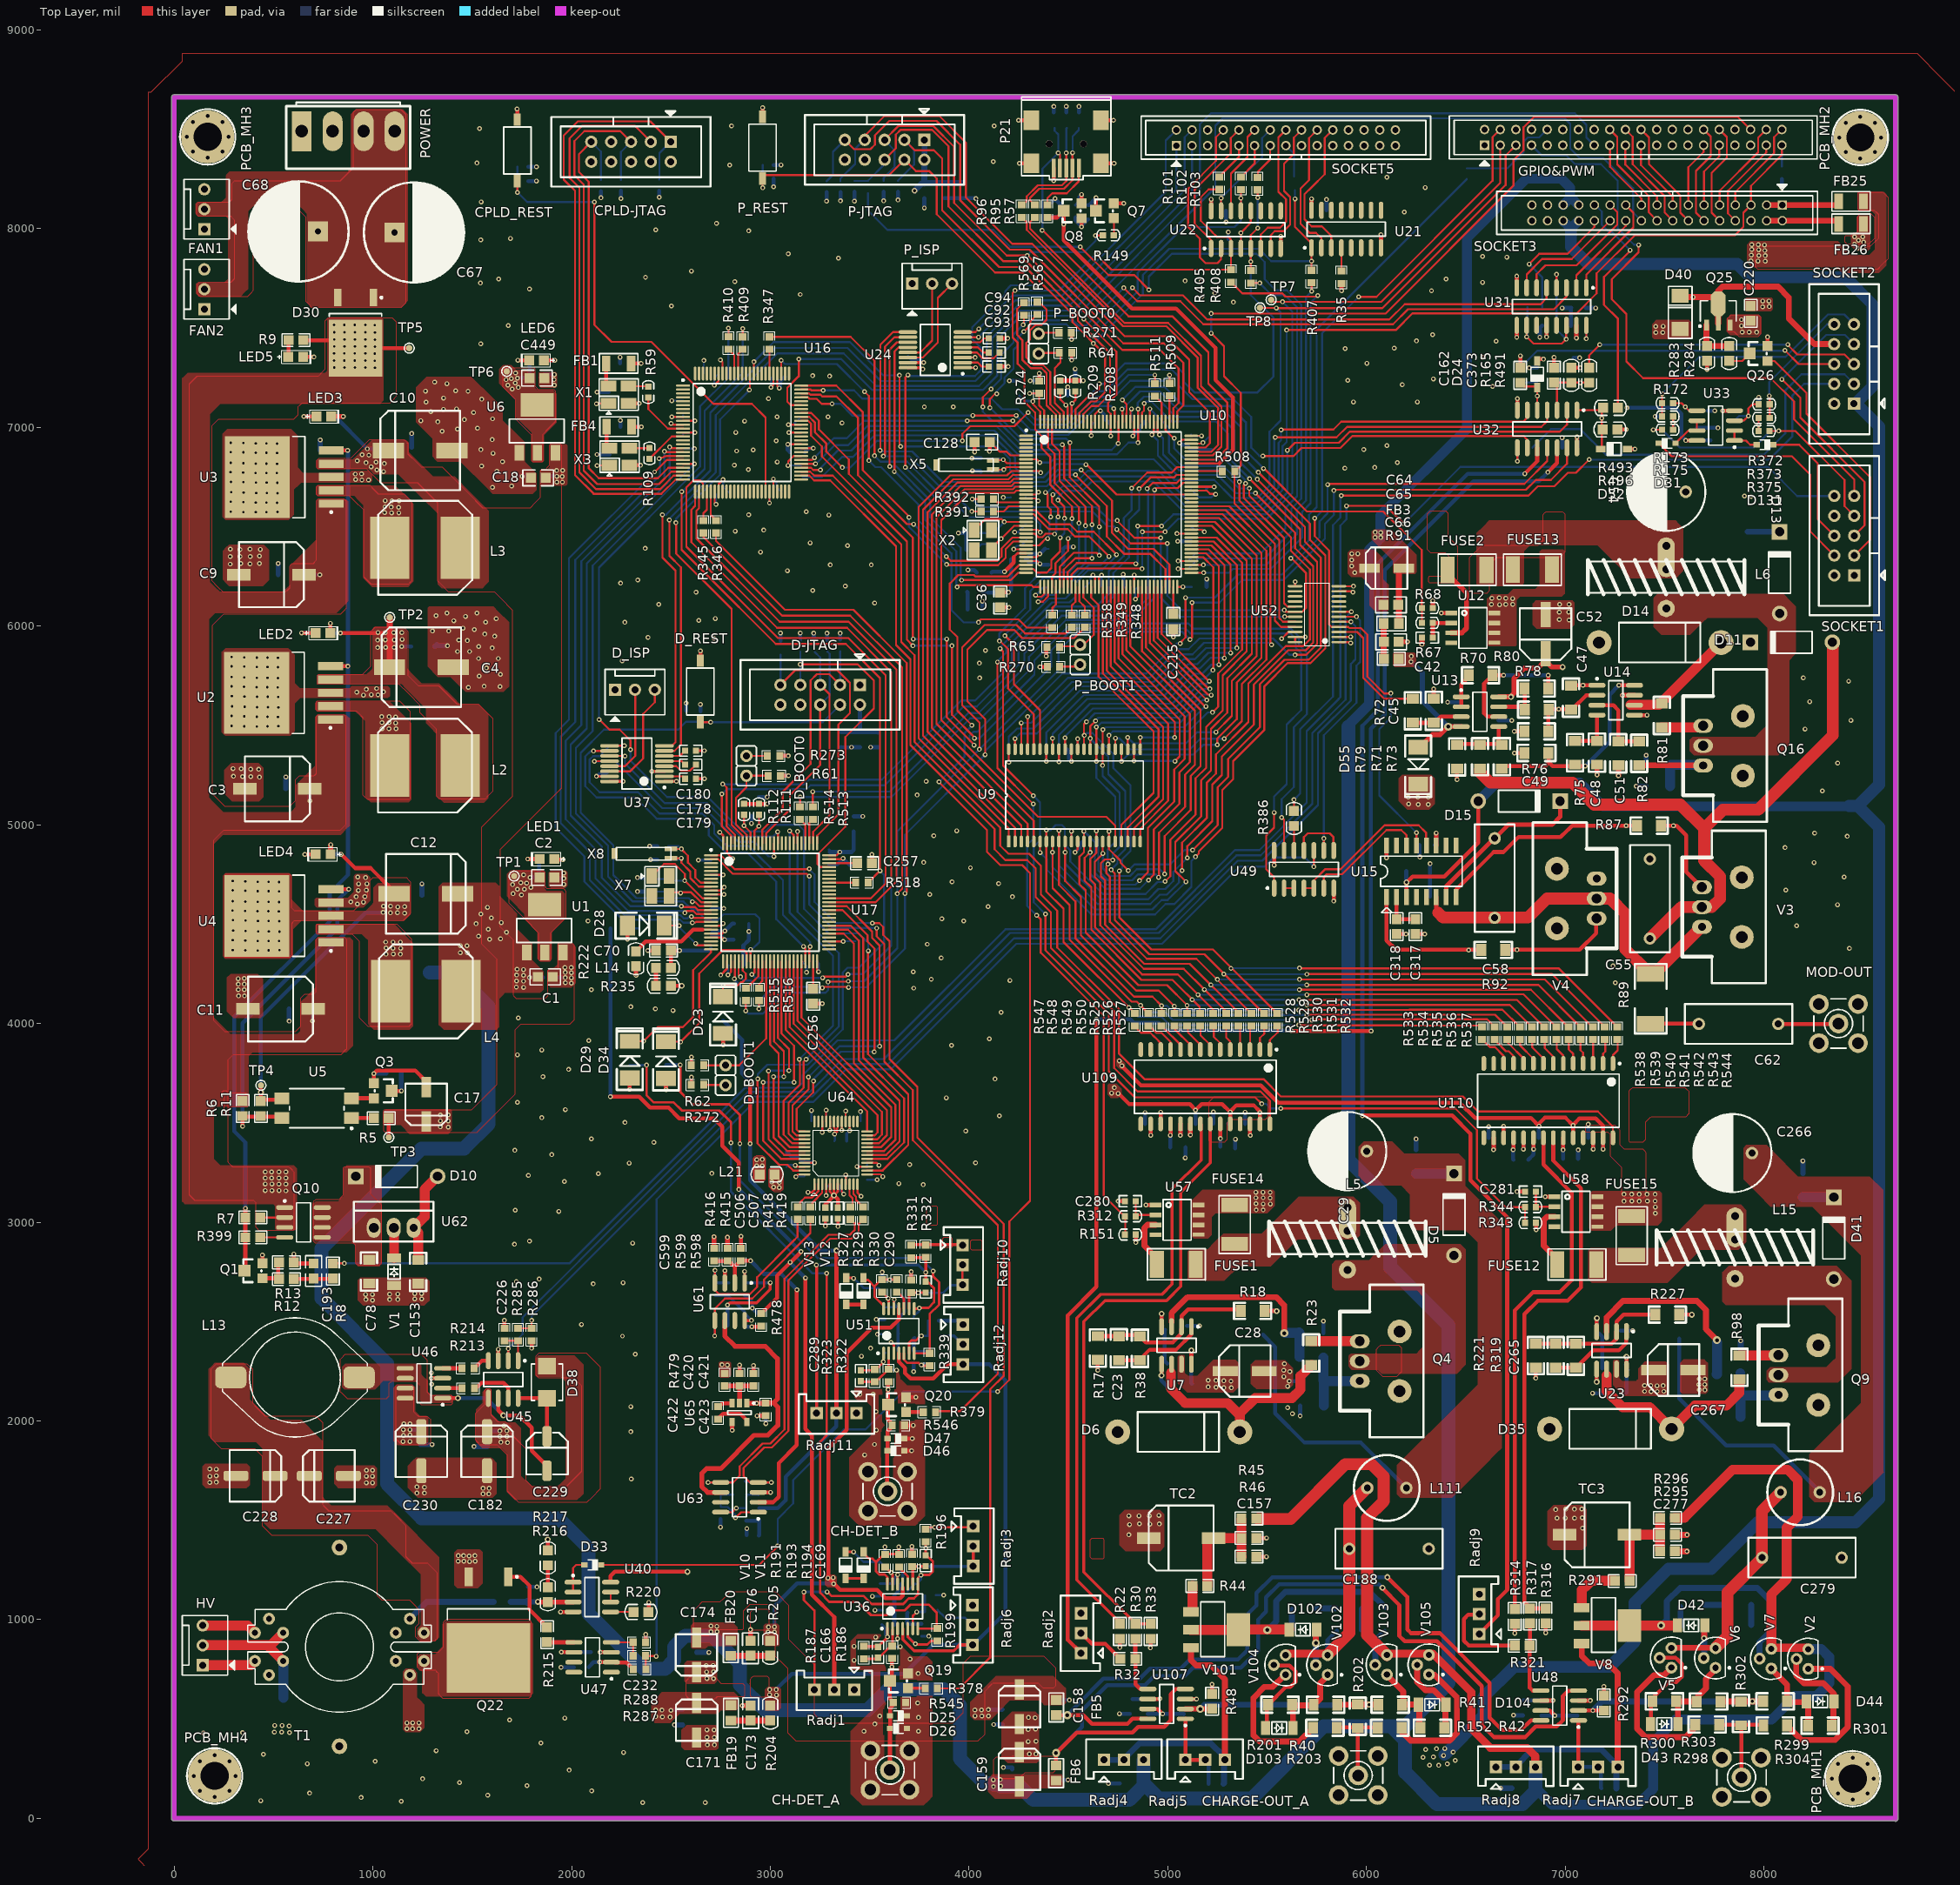
[diagram p0: Top Layer view]
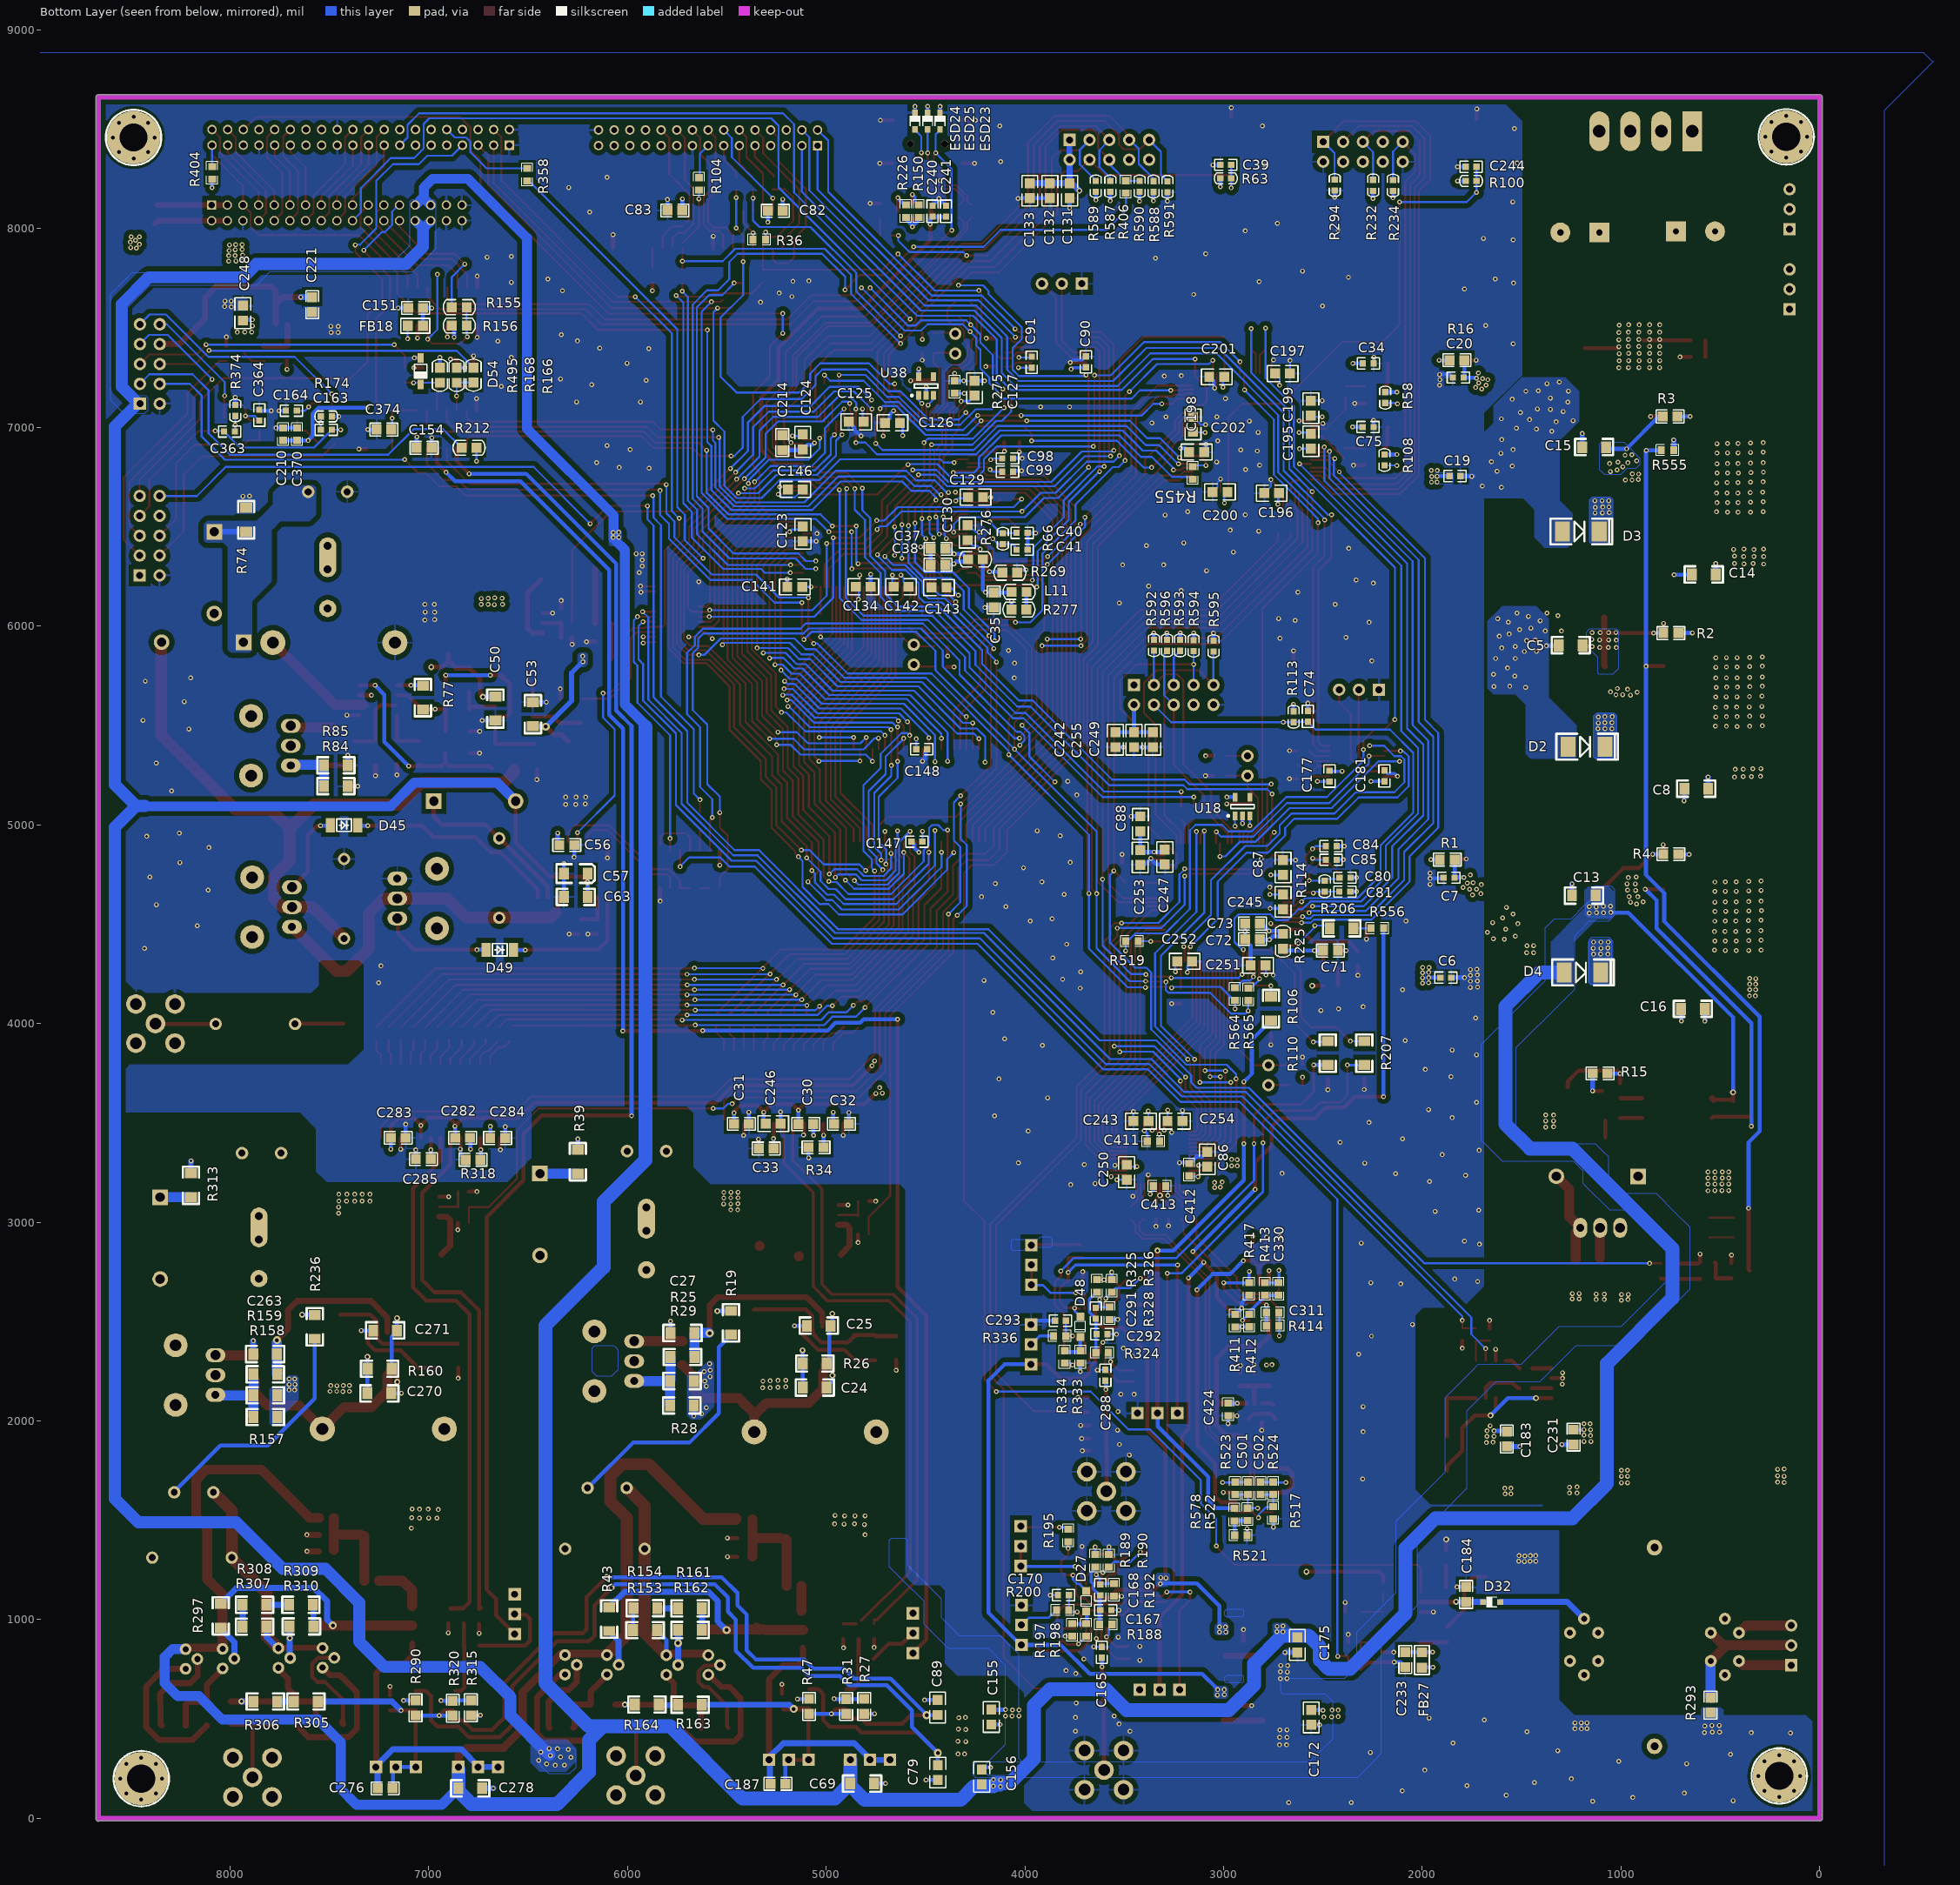
[diagram p1: Bottom Layer view, seen from below]
# Altium PCB MISC82309.PcbDoc (part 1 of 14)
Units mil, origin at the board's own origin, x right, y up, seen from the top; angles counter-clockwise.
Board outline 8687.03 x 8687.86 mil, 4 copper layers (Top Layer, GND, POWER, Bottom Layer); 747 components, 583 nets, 2530 pads, 1834 vias.

## Layer stack, top to bottom (the 12.6 mil dielectric is the usual default, probably not edited)
Top Layer: signal copper 1.4
Dielectric: core 12.6, FR-4, Dk 4.8
GND: plane copper 1.4, net GND
Dielectric: prepreg 12.6, FR-4, Dk 4.8
POWER: plane copper 1.4, net (Multiple Nets)
Dielectric: core 12.6, FR-4, Dk 4.8
Bottom Layer: signal copper 1.4

## Board outline
0,-12.51 cw(c0,0) -12.51,0 -12.51,8661.42 cw(c0,8661.42) 0,8673.93 8661.42,8673.93 cw(c8661.42,8661.42) 8673.26,8665.46 cw(c8662,8660) 8674.51,8660 8674.51,-1.42 cw(c8662,-1.42) 8656.22,-12.51

## Design rules (kind name [scope] priority, off if disabled: settings)
Clearance Clearance_1 [inpolygon] p1: gap=7
Clearance [All] p2: gap=7
DiffPairsRouting [All] p1: maxlimit=10 minlimit=10 mostfreqgap=10 maxuncoupledlength=500
Height [All] p1: minheight=0 maxheight=5000 prefheight=500
HoleSize [All] p1: absolutevalues=TRUE maxlimit=500 minlimit=1 maxpercent=80.000 minpercent=20.000
MinimumSolderMaskSliver [All] p1: minsoldermaskwidth=0
PlaneClearance [All] p1: clearance=20
PlaneConnect [All] p1: planeconnectstyle=Direct reliefexpansion=20 reliefentries=4 reliefconductorwidth=10 reliefairgap=10
PolygonConnect PolygonConnect_1 [All vs isvia] p1: connectstyle=Direct reliefconductorwidth=10 reliefentries=4 polygonreliefangle="90 Angle"
PolygonConnect [All] p2: connectstyle=Relief reliefconductorwidth=10 reliefentries=4 polygonreliefangle="90 Angle"
RoutingVias [All] p1: holewidth=12 width=24 viastyle="Through Hole" minholewidth=12 minwidth=24 maxholewidth=20 maxwidth=40
SilkToSilkClearance [All] p1: silktosilkclearance=0
SilkscreenOverComponentPads [IsPad] p1: minsilkscreentomaskgap=0
SolderMaskExpansion [All] p1: expansion=4
Width [All] p1: maxlimit=100 minlimit=10 preferedwidth=10 minimp=50.000000 maximp=50.000000 favimp=50.000000
20 further rules are at their usual default settings.

## Classes and differential pairs
component class PRINTING_CHARGE_A: C23 C24 C25 C27 C28 C29 C30 C31 C32 C33 C69 C79 C89 C155 C156 C157 C158 C159 C187 C188 C280 CHARGE-OUT_A D5 D6 D102 D103 D104 FB5 FB6 FUSE1 FUSE14 L5 L111 Q4 R17 R18 R19 R22 R23 R25 R26 R27 R28 R29 R30 R31 R32 R33 R34 R38 R39 R40 R41 R42 R43 R44 R45 R46 R47 R48 R151 R152 R153 R154 R161 R162 R163 R164 R201 R202 R203 R312 Radj2 Radj4 Radj5 TC2 U7 U57 U107 U109 V101 V102 V103 V104 V105
component class PRINTING_CHARGE_B: C263 C265 C266 C267 C270 C271 C276 C277 C278 C279 C281 C282 C283 C284 C285 CHARGE-OUT_B D35 D41 D42 D43 D44 FUSE12 FUSE15 L15 L16 Q9 R98 R157 R158 R159 R160 R221 R227 R236 R290 R291 R292 R295 R296 R297 R298 R299 R300 R301 R302 R303 R304 R305 R306 R307 R308 R309 R310 R313 R314 R315 R316 R317 R318 R319 R320 R321 R343 R344 Radj7 Radj8 Radj9 TC3 U23 U48 U58 U110 V2 V5 V6 V7 V8
component class PRINTING_CHARGEDETECT_A: C165 C166 C167 C168 C169 C170 C171 C172 C173 C174 C175 C176 C311 C330 C411 C412 C413 C506 C507 C599 CH-DET_A D25 D26 D27 FB19 FB20 L21 Q19 R186 R187 R188 R189 R190 R191 R192 R193 R194 R195 R196 R197 R198 R199 R200 R204 R205 R378 R411 R412 R413 R414 R415 R416 R417 R418 R419 R478 R545 R556 R598 R599 Radj1 Radj3 Radj6 U36 U61 U64 V10 V11
component class PRINTING_CHARGEDETECT_B: C288 C289 C290 C291 C292 C293 C420 C421 C422 C423 C424 C501 C502 CH-DET_B D46 D47 D48 Q20 R322 R323 R324 R325 R326 R327 R328 R329 R330 R331 R332 R333 R334 R336 R339 R379 R479 R517 R521 R522 R523 R524 R546 R578 Radj10 Radj11 Radj12 U51 U63 U65 V12 V13
component class PRINTING_CONNECT: C82 C83 C90 C91 C92 C93 C94 C177 C178 C179 C180 C181 D_BOOT0 D_BOOT1 D_ISP FB25 FB26 GPIO&PWM P_BOOT0 P_BOOT1 P_ISP R35 R36 R61 R62 R64 R65 R101 R102 R103 R104 R270 R271 R272 R273 R358 R404 SOCKET1 SOCKET2 SOCKET3 SOCKET5 TP7 TP8 U21 U22 U24 U37
component class PRINTING_CPLD: C34 C75 C195 C196 C197 C198 C199 C200 C201 C202 C244 CPLD-JTAG CPLD_REST FB1 FB4 R58 R59 R100 R108 R109 R232 R234 R294 R345 R346 R347 R409 R410 R455 R558 U16 X1 X3
component class PRINTING_HV: C182 C183 C184 C226 C227 C228 C229 C230 C231 C232 C233 D32 D33 D38 FB27 HV L13 Q22 R213 R214 R215 R216 R217 R220 R285 R286 R287 R288 R293 T1 U40 U45 U46 U47
component class PRINTING_MCU_DECTECT: C70 C71 C72 C73 C74 C80 C81 C84 C85 C86 C87 C88 C242 C243 C245 C246 C247 C248 C249 C250 C251 C252 C253 C254 C255 C256 C257 D23 D28 D29 D34 D-JTAG D_REST L14 R106 R110 R111 R112 R113 R114 R206 R207 R222 R225 R235 R513 R514 R515 R516 R518 R519 R564 R565 R592 R593 R594 R595 R596 U17 U18 X7 X8
component class PRINTING_MCU_PROCESSOR: C35 C36 C37 C38 C39 C40 C41 C98 C99 C123 C124 C125 C126 C127 C128 C129 C130 C131 C132 C133 C134 C141 C142 C143 C146 C214 C215 C240 C241 ESD23 ESD24 ESD25 L11 P21 P-JTAG P_REST Q7 Q8 R57 R63 R66 R95 R96 R149 R150 R208 R209 R226 R269 R274 R275 R276 R277 R348 R349 R391 R392 R405 R406 R407 R408 R508 R509 R511 R567 R569 R587 R588 R589 R590 R591 U10 U38 X2 X5
component class PRINTING_MODULATION: C42 C45 C47 C48 C49 C50 C51 C52 C53 C54 C55 C56 C57 C58 C62 C63 C64 C65 C66 C317 C318 D11 D13 D14 D15 D45 D49 D55 FB3 FUSE2 FUSE13 L6 MOD-OUT Q16 R67 R68 R70 R71 R72 R73 R74 R75 R76 R77 R78 R79 R80 R81 R82 R84 R85 R87 R89 R91 R92 U12 U13 U14 U15 U49 U52 V3 V4
component class PRINTING_SYNCHRONIZER: C151 C154 C162 C163 C164 C210 C220 C221 C363 C364 C370 C373 C374 D24 D31 D40 D52 D54 D131 FB18 Q25 Q26 R155 R156 R165 R166 R168 R172 R173 R174 R175 R212 R283 R284 R372 R373 R374 R375 R386 R491 R493 R495 R496 U31 U32 U33
component class SYSTEM_POWER: C1 C2 C3 C4 C5 C6 C7 C8 C9 C10 C11 C12 C13 C14 C15 C16 C17 C18 C19 C20 C67 C68 C78 C153 C193 C449 D2 D3 D4 D10 D30 FAN1 FAN2 L2 L3 L4 LED1 LED2 LED3 LED4 LED5 LED6 PCB_MH1 PCB_MH2 PCB_MH3 PCB_MH4 POWER Q1 Q3 Q10 R1 R2 R3 R4 R5 R6 R7 R8 R9 R11 R12 R13 R15 R16 R399 R555 TP1 TP2 TP3 TP4 TP5 TP6 U1 U2 U3 U4 U5 U6 U62 V1
net class D_A[0..11]: D_A0 D_A1 D_A2 D_A3 D_A4 D_A5 D_A6 D_A7 D_A8 D_A9 D_A10 D_A11
net class D_B[0..11]: D_B0 D_B1 D_B2 D_B3 D_B4 D_B5 D_B6 D_B7 D_B8 D_B9 D_B10 D_B11
net class DET_D[0..15]: DET_D0 DET_D1 DET_D2 DET_D3 DET_D4 DET_D5 DET_D6 DET_D7 DET_D8 DET_D9 DET_D10 DET_D11 DET_D12 DET_D13 DET_D14 DET_D15
net class FSMC_A[0..25]: FSMC_A0 FSMC_A1 FSMC_A2 FSMC_A3 FSMC_A4 FSMC_A5 FSMC_A6 FSMC_A7 FSMC_A8 FSMC_A9 FSMC_A10 FSMC_A11 FSMC_A12 FSMC_A13 FSMC_A14 FSMC_A15 FSMC_A16 FSMC_A17 FSMC_A18 FSMC_A19 FSMC_A20 FSMC_A21 FSMC_A22 FSMC_A23 FSMC_A24 FSMC_A25
net class FSMC_D[0..15]: FSMC_D0 FSMC_D1 FSMC_D2 FSMC_D3 FSMC_D4 FSMC_D5 FSMC_D6 FSMC_D7 FSMC_D8 FSMC_D9 FSMC_D10 FSMC_D11 FSMC_D12 FSMC_D13 FSMC_D14 FSMC_D15
component class PRINTING_RAM: C147 C148 R525 R526 R527 R528 R529 R530 R531 R532 R533 R534 R535 R536 R537 R538 R539 R540 R541 R542 R543 R544 R547 R548 R549 R550 U9
differential pair NewDifferentialPair1: +OUT- -OUT+

## Components (designator, comment, footprint, x,y, rotation, side; value= is the part's Value field where it differs from the comment)
C1 "22uF" C0805 1868,4235 r0 top
C2 "22uF" C0805 1876,4735 r180 top
C3 "220uF/35V" E8X10,2 683,5181 r180 top
C4 "470uF/25V" E10X10.2 1084,5793 r0 top
C5 "0.1uF" C1206 1253,5903 r0 bottom
C6 "0.1uF" C0603 1882,4231 r0 bottom
C7 "0.1uF" C0603 1866,4734 r180 bottom
C8 "0.1uF" C1206 622,5181 r0 bottom
C9 "220uF/35V" E8X10,2 653,6259 r180 top
C10 "470uF/25V" E10X10.2 1078,6884 r0 top
C11 "220uF/35V" E8X10,2 699,4073 r180 top
C12 "470uF/25V" E10X10.2 1427,4653 r180 top
C13 "0.1uF" C1206 1187,4645 r180 bottom
C14 "0.1uF" C1206 584,6259 r0 bottom
C15 "0.1uF" C1206 1136,6900 r0 bottom
C16 "0.1uF" C1206 639,4073 r0 bottom
C17 "47uF/16V" E5X5.4 1269,3507 r90 top
C18 "22uF" C0805 1832,6746 r0 top
C19 "0.1uF" C0603 1836,6755 r0 bottom
C20 "0.1uF" C0603 1819,7251 r180 bottom
C23 "47pF" C1206 4755,2366 r270 top
C24 "10nF" C1206 5057,2169 r180 bottom
C25 "2.2nF" C1206 5037,2479 r0 bottom
C27 "470pF" C1206 5723,2442 r0 bottom
C28 "22uF/35V" E6.3X5.4 5289,2251 r0 top
C29 "2.2uF/450V" CAP-EL-10X13_5-5 5903,3358 r0 top
C30 "0.1uF" CAP_0805 5102,3494 r180 bottom
C31 "0.1uF" CAP_0805 5426,3495 r180 bottom
C32 "0.1uF" CAP_0805 4923,3495 r180 bottom
C33 "0.1uF" CAP_0805 5301,3371 r180 bottom
C34 "0.1uF" C0603 2272,7322 r0 bottom
C35 "1uF" CAP_0805 4157,6131 r90 bottom
C36 "0.1uF" CAP_0805 4157,6131 r90 top
C37 "1uF" CAP_0805 4437,6389 r180 bottom
C38 "0.1uF" CAP_0805 4437,6309 r180 bottom
C39 "0.1uF" C0603 2989,8321 r180 bottom
C40 "20pF" C0603 4014,6469 r0 bottom
C41 "20pF" C0603 4014,6384 r0 bottom
C42 "470pF" C0603 6306,5942 r0 top
C45 "0.22uF" c1206 6338,5574 r90 top
C47 "47pF" C1206 7030,5640 r270 top
C48 "2.2nF" C1206 7160,5363 r270 top
C49 "10nF" C1206 6855,5361 r180 top
C50 "0.47uF" c1206 6664,5585 r270 bottom
C51 "470pF" C1206 7268,5360 r270 top
C52 "22uF/35V" E6.3X5.4 6901,5861 r90 top
C53 "0.47uF" c1206 6476,5557 r90 bottom
C54 "2.2uF/450V" CAP-EL-10X13_5-5 7508,6676 r0 top
C55 "0.33uF/400V" CBB-400V-10mm 7426,4628 r270 top
C56 "0.1uF" CAP_0805 6305,4898 r180 bottom
C57 "22uF/35V" CAP_AVX-A 6260,4755 r0 bottom
C58 "0.1uF/400V" CBB-400V-10mm 6645,4732 r90 top
C62 "22nF/630V" CBB-400V-10mm 7872,3998 r0 top
C63 "0.1uF" C1206 6260,4638 r180 bottom
C64 "10uF/25V" E5X5.4 6015,6291 r0 top
C65 "0.1uF" C0805 6123,6107 r0 top
C66 "0.1uF" C0805 6124,5921 r180 top
C67 "1000uF/35V" CAP-EL-12x20 1207,7981 r0 top
C68 "1000uF/35V" CAP-EL-12x20 626,7986 r180 top
C69 "0.47uF" C1206 4819,176 r180 bottom
C70 "1uF" CAP_0805 2462,4367 r0 top
C71 "0.1uF" CAP_0805 2462,4367 r0 bottom
C72 "1uF" CAP_0805 2855,4425 r180 bottom
C73 "0.1uF" CAP_0805 2855,4503 r180 bottom
C74 "0.1uF" C0603 2576,5546 r270 bottom
C75 "0.1uF" C0603 2273,7002 r0 bottom
C78 "0.33uF" c1206 982,2752 r270 top
C79 "0.1uF" C0805 4438,231 r90 bottom
C80 "20pF" C0603 2389,4734 r0 bottom
C81 "20pF" C0603 2390,4664 r0 bottom
C82 "0.1uF" CAP_0805 5256,8090 r180 bottom
C83 "0.1uF" CAP_0805 5761,8092 r180 bottom
C84 "10pF" C0603 2459,4893 r0 bottom
C85 "10pF" C0603 2459,4824 r0 bottom
C86 "100nF" C0805 3082,3317 r270 bottom
C87 "100nF" C0805 2701,4785 r270 bottom
C88 "100nF" C0805 3419,5005 r270 bottom
C89 "0.1uF" C0805 4439,558 r270 bottom
C90 "0.1uF" C0603 3693,7330 r270 bottom
C91 "0.1uF" C0603 3966,7328 r270 bottom
C92 "0.1uF" C0603 4126,7377 r0 top
C93 "0.1uF" C0603 4126,7306 r180 top
C94 "0.1uF" C0603 4127,7448 r180 top
C98 "10pF" C0603 4087,6844 r0 bottom
C99 "10pF" C0603 4087,6777 r0 bottom
C123 "10uF" C0805 5117,6464 r90 bottom
C124 "100nF" C0805 5118,6927 r90 bottom
C125 "10uF" C0805 4849,7028 r180 bottom
C126 "100nF" C0805 4666,7023 r180 bottom
C127 "10uF" C0805 4253,7197 r270 bottom
C128 "100nF" C0805 4066,6926 r0 top
C129 "10uF" C0805 4248,6649 r0 bottom
C130 "100nF" C0805 4289,6470 r270 bottom
C131 "10uF" C0805 3775,8191 r90 bottom
C132 "100nF" C0805 3874,8191 r90 bottom
C133 "10uF" C0805 3975,8191 r90 bottom
C134 "100nF" C0805 4813,6198 r0 bottom
C141 "10uF" C0805 5158,6197 r180 bottom
C142 "100nF" C0805 4623,6198 r0 bottom
C143 "10uF" C0805 4432,6194 r0 bottom
C146 "100nF" C0805 5155,6688 r0 bottom
C147 "100nF" C0603 4543,4915 r180 bottom
C148 "100nF" C0603 4519,5381 r0 bottom
C151 "0.1uF" CAP_0805 7066,7601 r180 bottom
C153 "0.1uF" c1206 1229,2750 r270 top
C154 "0.1uF" CAP_0805 7023,6897 r0 bottom
C155 "100nF" C0805 4169,510 r270 bottom
C156 "100nF" C0805 4217,209 r90 bottom
C157 "0.1uF" CAP_0805 5408,1317 r0 top
C158 "10uF/25V" E5X5.4 4253,648 r270 top
C159 "10uF/25V" E5X5.4 4253,333 r270 top
C162 "0.1uF" CAP_0805 6774,7262 r270 top
C163 "0.47uF" C0603 7515,6988 r180 bottom
C164 "330pF" C0603 7691,7084 r180 bottom
C165 "470pF" C0603 3613,836 r270 bottom
C166 "1.5nF" C0603 3542,836 r270 top
C167 "0.01uF" C0603 3593,1048 r180 bottom
C168 "0.01uF" C0603 3621,1150 r270 bottom
C169 "1.5nF" C0603 3782,1297 r270 top
C170 "0.22uF" C0603 3806,1124 r0 bottom
C171 "10uF/25V" E5X5.4 2629,580 r270 top
C172 "0.1uF" C0805 2559,508 r90 bottom
C173 "0.1uF" C0805 2901,530 r270 top
C174 "10uF/25V" E5X5.4 2629,737 r90 top
C175 "0.1uF" C0805 2629,873 r90 bottom
C176 "0.1uF" C0805 2900,856 r270 top
C177 "0.1uF" C0603 2467,5245 r270 bottom
C178 "0.1uF" C0603 2599,5303 r0 top
C179 "0.1uF" C0603 2599,5232 r180 top
C180 "0.1uF" C0603 2599,5373 r180 top
C181 "0.1uF" C0603 2191,5246 r270 bottom
C182 "22uF/35V" CAP-ALU-6_3X5_4 1575,1946 r270 top
C183 "0.1uF" CAP_0805 1575,1909 r90 bottom
C184 "0.1uF" CAP_0805 1780,1127 r270 bottom
C187 "0.22nF" CAP_0805 5242,174 r180 bottom
C188 "0.33uF/400V" CBB-400V-10mm 6113,1357 r180 top
C193 "10uF" C0805 702,2755 r270 top
C195 "10nF" C0805 2561,6930 r90 bottom
C196 "100nF" C0805 2758,6669 r180 bottom
C197 "10nF" C0805 2703,7271 r0 bottom
C198 "100nF" C0805 3136,6876 r0 bottom
C199 "10nF" C0805 2561,7097 r270 bottom
C200 "100nF" C0805 3018,6675 r180 bottom
C201 "10nF" C0805 3035,7254 r180 bottom
C202 "100nF" C0805 3154,7015 r270 bottom
C210 "0.1uF" CAP_0603 7732,6966 r270 bottom
C214 "2.2uF" CAP_0805 5221,6923 r270 bottom
C215 "2.2uF" CAP_0805 5028,6023 r270 top
C220 "10uF" CAP_0805 7933,7574 r270 top
C221 "10uF" CAP_0805 7586,7618 r90 bottom
C226 "0.1uF" CAP_0603 1662,2435 r270 top
C227 "33uF/35V" CAP-ALU-6_3X5_4 680,1724 r0 top
C228 "33uF/35V" CAP-ALU-6_3X5_4 508,1724 r180 top